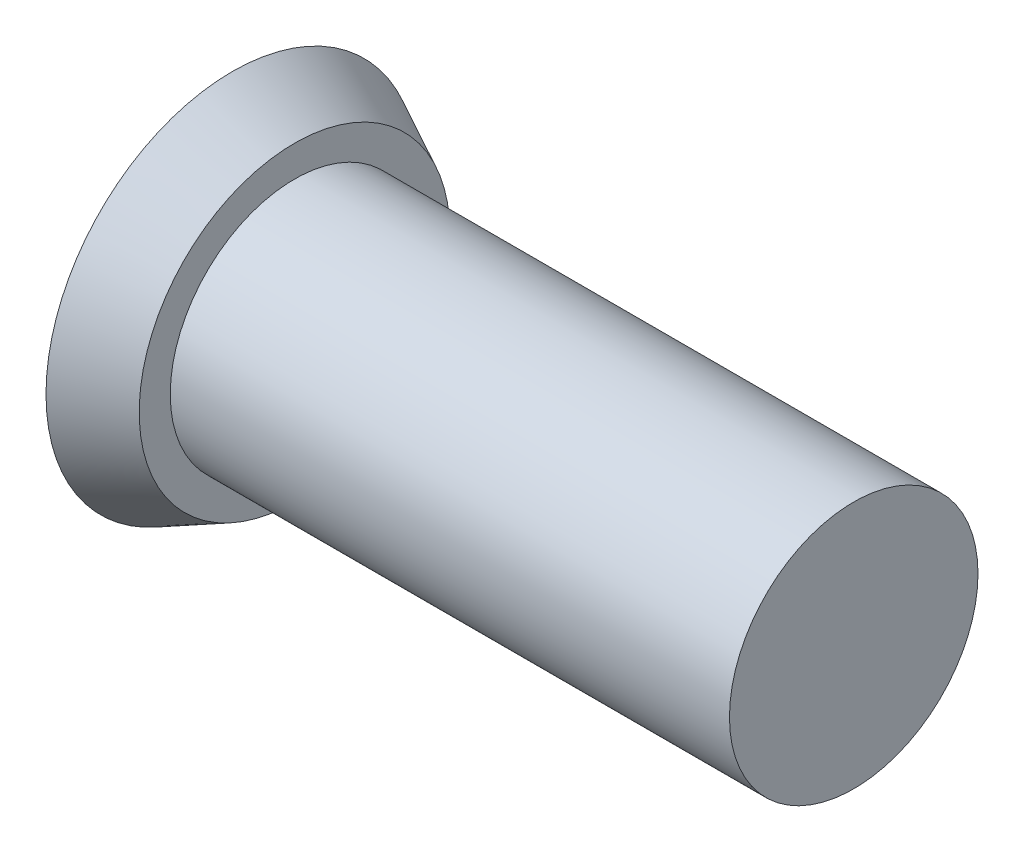
from build123d import *


with BuildPart() as part:
    # Sketch1 → Revolve1 (revolve)
    with BuildSketch(Plane.XY, mode=Mode.PRIVATE) as revolve1_sk:
        Polygon((0, 0), (0, 3), (1, 2.5), (1, 2), (10, 2), (10, 0), align=None)
    revolve(revolve1_sk.sketch.rotate(Axis((10, 0, 0), (-1, 0, 0)), 90), axis=Axis((10, 0, 0), (-1, 0, 0)))


solid = part.part
